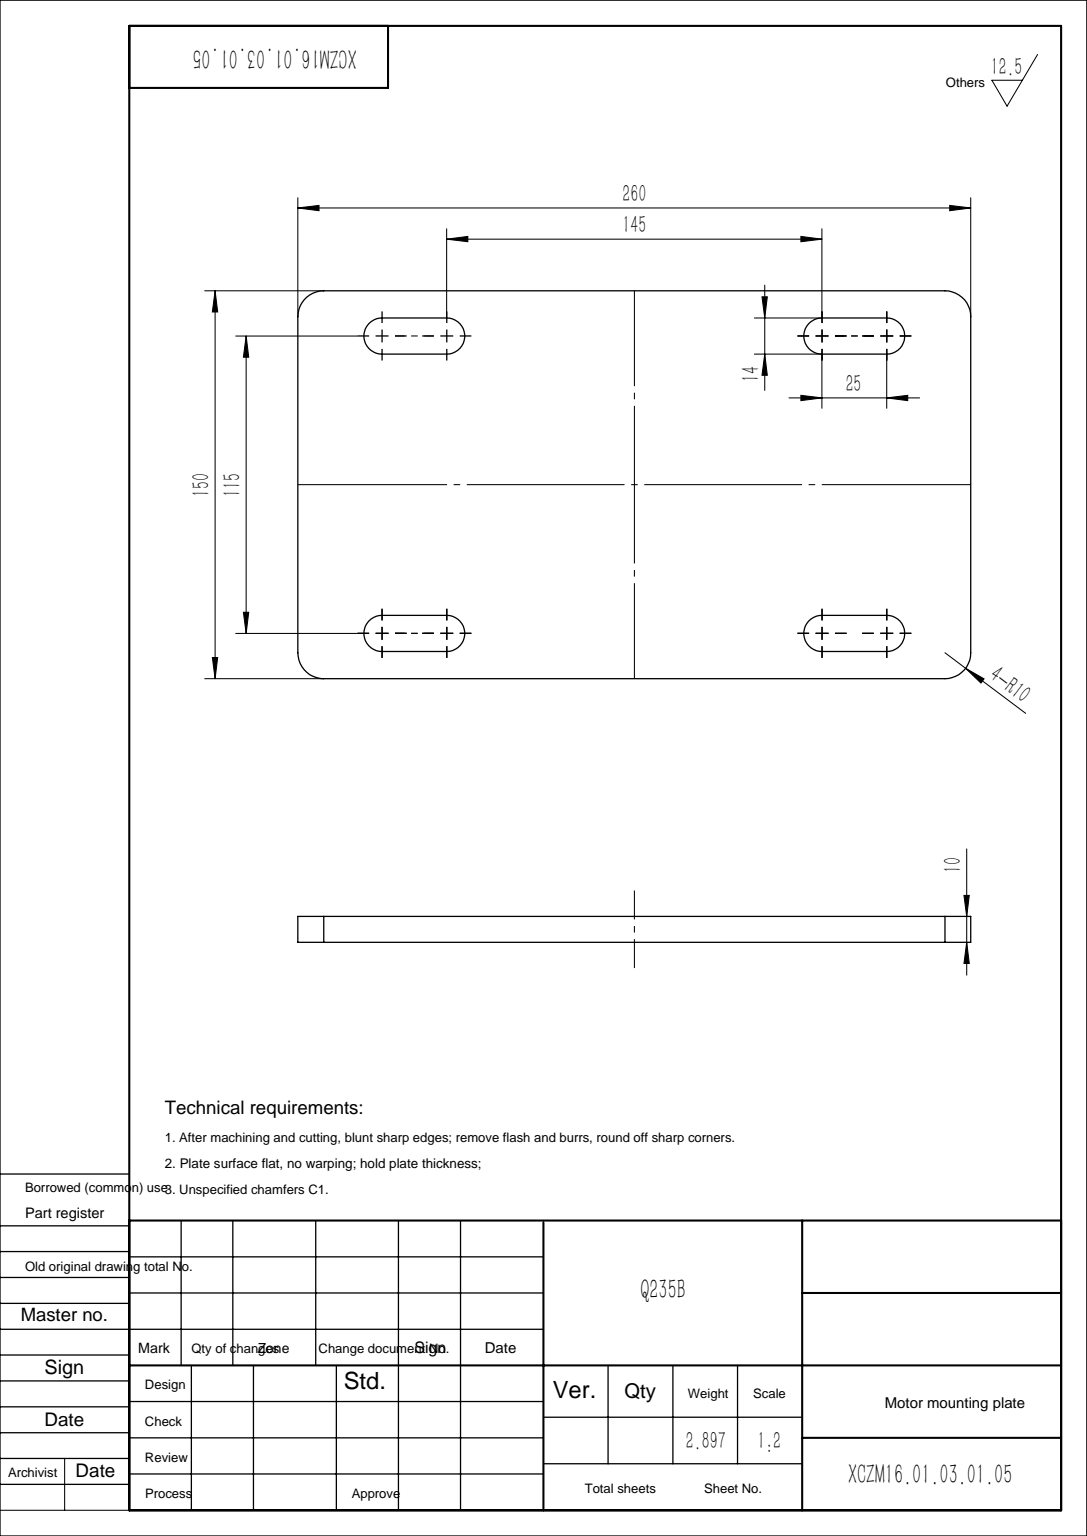
SolidWorks part; units mm, degrees
material "XRAAT"
ref_plane "前视基准面" through (0, 0, 0) normal (0, 0, 1) x (1, 0, 0)
ref_plane "上视基准面" through (0, 0, 0) normal (0, 1, 0) x (1, 0, 0)
ref_plane "右视基准面" through (0, 0, 0) normal (1, 0, 0) x (0, 0, -1)
sketch "草图1" plane through (0, 0, 0) normal (0, 1, 0) x (1, 0, 0)
  line L0 (-72.5, 57.5) -> (-97.5, 57.5) construction
  line L1 (120, -75) -> (-120, -75)
  line L2 (130, -65) -> (130, 65)
  line L3 (120, 75) -> (-120, 75)
  line L4 (-130, -65) -> (-130, 65)
  line L5 (130, -75) -> (-130, 75) construction
  line L6 (130, 75) -> (-130, -75) construction
  line L7 (-72.5, 50.5) -> (-97.5, 50.5)
  line L8 (-72.5, 64.5) -> (-97.5, 64.5)
  line L9 (0, 75) -> (0, 0) construction
  line L10 (0, 0) -> (-130, 0) construction
  line L11 (72.5, 57.5) -> (97.5, 57.5) construction
  line L12 (72.5, 50.5) -> (97.5, 50.5)
  line L13 (72.5, 64.5) -> (97.5, 64.5)
  line L14 (-72.5, -57.5) -> (-97.5, -57.5) construction
  line L15 (-72.5, -50.5) -> (-97.5, -50.5)
  line L16 (-72.5, -64.5) -> (-97.5, -64.5)
  line L17 (72.5, -57.5) -> (97.5, -57.5) construction
  line L18 (72.5, -50.5) -> (97.5, -50.5)
  line L19 (72.5, -64.5) -> (97.5, -64.5)
  arc A0 (-120, -75) -> (-130, -65) centre (-120, -65) cw
  arc A1 (130, 65) -> (120, 75) centre (120, 65) ccw
  arc A2 (120, -75) -> (130, -65) centre (120, -65) ccw
  arc A3 (-120, 75) -> (-130, 65) centre (-120, 65) ccw
  arc A4 (-72.5, 50.5) -> (-72.5, 64.5) centre (-72.5, 57.5) ccw
  arc A5 (-97.5, 64.5) -> (-97.5, 50.5) centre (-97.5, 57.5) ccw
  arc A6 (72.5, 50.5) -> (72.5, 64.5) centre (72.5, 57.5) cw
  arc A7 (97.5, 64.5) -> (97.5, 50.5) centre (97.5, 57.5) cw
  arc A8 (-72.5, -50.5) -> (-72.5, -64.5) centre (-72.5, -57.5) cw
  arc A9 (-97.5, -64.5) -> (-97.5, -50.5) centre (-97.5, -57.5) cw
  arc A10 (72.5, -50.5) -> (72.5, -64.5) centre (72.5, -57.5) ccw
  arc A11 (97.5, -64.5) -> (97.5, -50.5) centre (97.5, -57.5) ccw
  point P0 (0, 0)
  point P20 (-85, 57.5)
  point P30 (85, 57.5)
  point P37 (-85, -57.5)
  point P44 (85, -57.5)
  dimension "D3" = 10
  dimension "D1" = 150
  dimension "D2" = 260
  dimension "D4" = 25
  dimension "D5" = 14
  dimension "D6" = 145
  dimension "D7" = 115
extrude "凸台-拉伸1" add sketch "草图1" along normal blind 10
